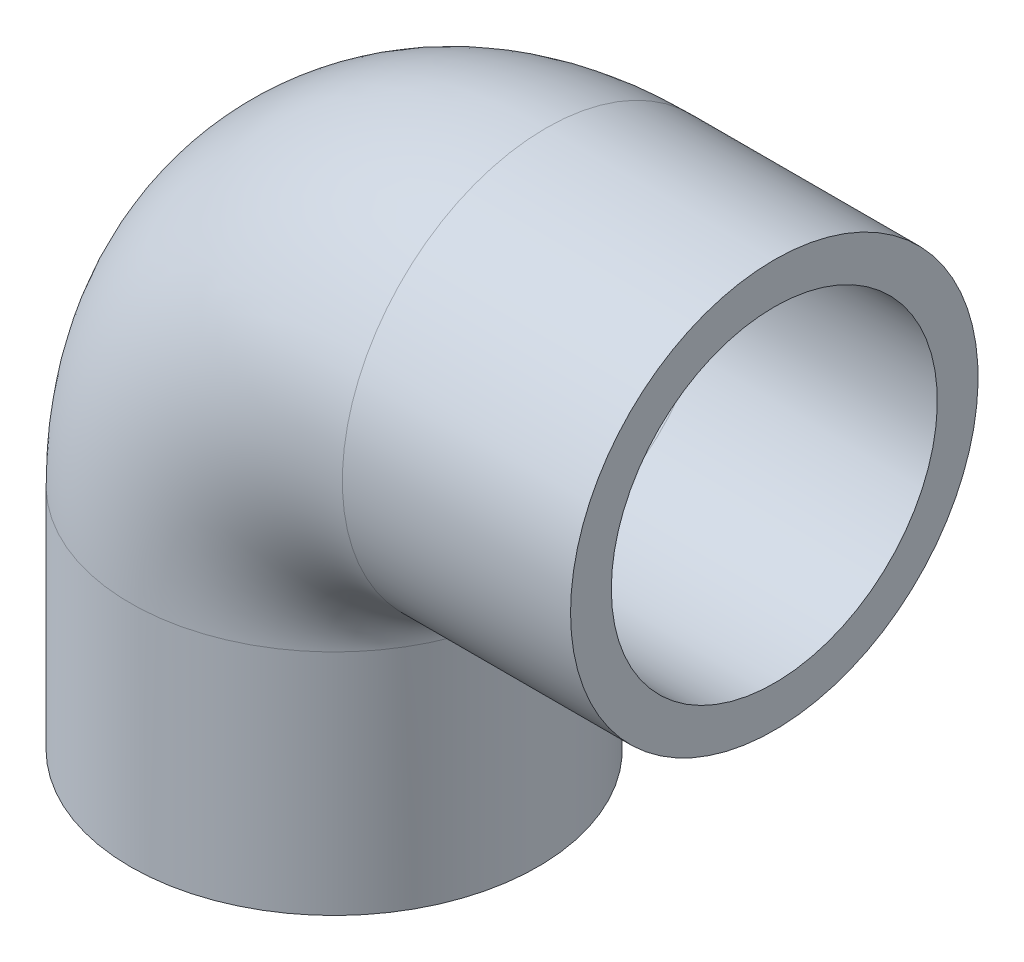
SolidWorks part; units mm, degrees
material "PP 共聚物"
ref_plane "前视基准面" through (0, 0, 0) normal (0, 0, 1) x (1, 0, 0)
ref_plane "上视基准面" through (0, 0, 0) normal (0, 1, 0) x (1, 0, 0)
ref_plane "右视基准面" through (0, 0, 0) normal (1, 0, 0) x (0, 0, -1)
sketch "草图1" plane through (0, 0, 0) normal (0, 0, 1) x (1, 0, 0)
  line L0 (0, 0) -> (0, 14)
  line L1 (13, 27) -> (27, 27)
  line L2 (27, 27) -> (0, 27) construction
  line L3 (0, 27) -> (0, 0) construction
  line L4 (10, 0) -> (12.5, 0) construction
  arc A0 (0, 14) -> (13, 27) centre (13, 14) cw
  dimension "D2" = 14
  dimension "a1" = 27
  dimension "dn1" = 20
  dimension "d1" = 25
sketch "草图2" plane through (0, 0, 0) normal (0, 1, 0) x (1, 0, 0)
  circle A0 centre (0, 0) radius 10
  circle A1 centre (0, 0) radius 12.5
sweep "扫描1" add profiles "草图2" path "草图1"
